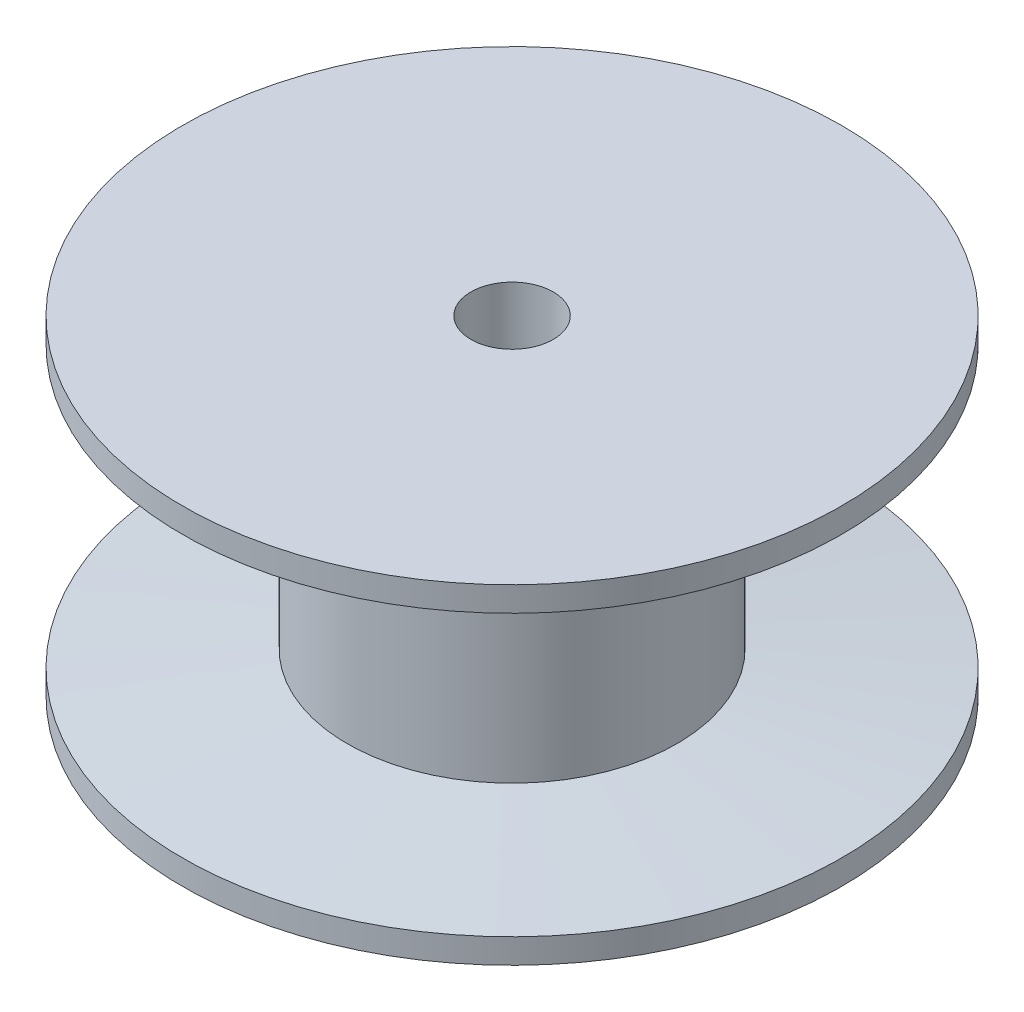
SolidWorks part; units mm, degrees
ref_plane "前视基准面" through (0, 0, 0) normal (0, 0, 1) x (1, 0, 0)
ref_plane "上视基准面" through (0, 0, 0) normal (0, 1, 0) x (1, 0, 0)
ref_plane "右视基准面" through (0, 0, 0) normal (1, 0, 0) x (0, 0, -1)
sketch "草图1" plane through (0, 0, 0) normal (1, 0, 0) x (0, 0, -1)
  line L0 (0, 0) -> (0, 65.8261) construction
  line L1 (5, 0) -> (40, 0)
  line L3 (40, 0) -> (40, 3)
  line L6 (20, 5) -> (40, 3)
  line L7 (20, 5) -> (20, 35)
  line L10 (40, 37) -> (20, 35)
  line L11 (40, 37) -> (40, 40)
  line L12 (40, 40) -> (5, 40)
  line L14 (5, 40) -> (5, 0)
revolve "旋转1" add sketch "草图1" angle 360 about L0
